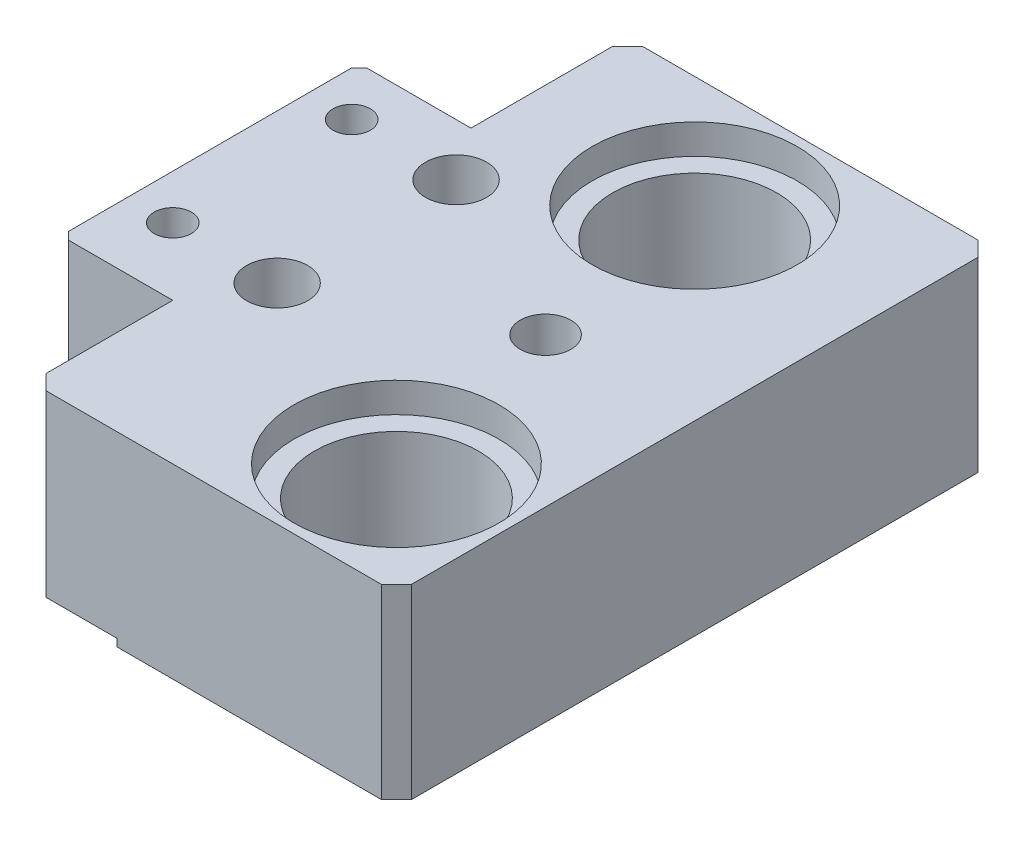
SolidWorks part; units mm, degrees
ref_plane "Front Plane" through (0, 0, 0) normal (0, 0, 1) x (1, 0, 0)
ref_plane "Top Plane" through (0, 0, 0) normal (0, 1, 0) x (1, 0, 0)
ref_plane "Right Plane" through (0, 0, 0) normal (1, 0, 0) x (0, 0, -1)
sketch "Sketch1" plane through (0, 0, 0) normal (0, 0, 1) x (1, 0, 0)
  line L0 (0, 91.2981) -> (0, -100.4583) construction
  line L1 (-32, 12.5) -> (32, 12.5)
  line L2 (-32, 12.5) -> (-32, -12.5)
  line L3 (-32, -12.5) -> (32, -12.5)
  line L4 (32, 12.5) -> (32, -12.5)
  line L5 (-125.8092, 0) -> (111.3632, 0) construction
  dimension "D1" = 64
  dimension "D2" = 25
extrude "Boss-Extrude1" add sketch "Sketch1" along normal mid plane 80
sketch "Sketch3" plane through (0, 12.5, 0) normal (0, 1, 0) x (1, 0, 0)
  line L0 (-32, -40) -> (32, -40) construction
  line L1 (32, -40) -> (32, 40) construction
  line L2 (-12, -12) -> (-12, 12) construction
  line L3 (-12, 0) -> (-32, 0) construction
  line L4 (-32, -40) -> (-32, 40) construction
  circle A0 centre (7, 25) radius 11
  circle A1 centre (17, -25) radius 11
  circle A2 centre (-12, 12) radius 2.5
  circle A3 centre (-12, -12) radius 2.5
  circle A4 centre (-26, 12) radius 2.5
  circle A5 centre (-26, -12) radius 2.5
  dimension "D1" = 22
  dimension "D2" = 15
  dimension "D3" = 15
  dimension "D4" = 22
  dimension "D5" = 10
  dimension "D6" = 50
  dimension "D8" = 5
  dimension "D10" = 6
  dimension "D7" = 24
  dimension "D9" = 20
extrude "Cut-Extrude1" cut sketch "Sketch3" against normal through all
hole_wizard "M3 Tapped Hole1" positions "Sketch5" profile "Sketch4" tap size "M3" standard "Gb"
sketch "Sketch5" plane through (-32, 0, 0) normal (-1, 0, 0) x (0, 0, 1)
  line L0 (0, -23.1259) -> (0, 24.6172) construction
  line L2 (40, -12.5) -> (-40, -12.5) construction
  point P0 (0, 3.5)
  point P1 (-6, -7.5)
  point P3 (6, -7.5)
  dimension "D1" = 5
  dimension "D2" = 11
  dimension "D3" = 12
sketch "Sketch4" plane through (-32, 3.5, 0) normal (0, 1, 0) x (0, 0, 1)
  line L0 (0, 0) -> (0, 8.2511)
  line L1 (0, 8.2511) -> (1.25, 7.5)
  line L2 (1.25, 7.5) -> (1.25, 0)
  line L5 (1.25, 0) -> (0, 0)
  line L10 (0, 8.2511) -> (-1.25, 7.5) construction
  line L11 (0, -6.35) -> (0, 107.95) construction
  dimension "螺纹孔钻头直径" = 2.5
  dimension "螺纹孔钻头深度" = 7.5
  dimension "导头角度" = 118
cosmetic thread "Hole cosmetic thread1" parameters "D1"=6, "D2"=3
cosmetic thread "Hole cosmetic thread2" parameters "D1"=6, "D2"=3
cosmetic thread "Hole cosmetic thread3" parameters "D1"=6, "D2"=3
hole_wizard "M8 Tapped Hole1" positions "Sketch8" profile "Sketch7" tap size "M8" standard "Gb"
sketch "Sketch8" plane through (0, 12.5, 0) normal (0, 1, 0) x (-1, 0, 0)
  line L0 (-32, 40) -> (-32, -40) construction
  point P0 (-12, 0)
  dimension "D1" = 20
sketch "Sketch7" plane through (12, 12.5, 0) normal (1, 0, 0) x (0, 0, 1)
  line L0 (0, 0) -> (0, 22.0429)
  line L1 (0, 22.0429) -> (3.4, 20)
  line L2 (3.4, 20) -> (3.4, 0)
  line L5 (3.4, 0) -> (0, 0)
  line L10 (0, 22.0429) -> (-3.4, 20) construction
  line L11 (0, -6.35) -> (0, 107.95) construction
  dimension "螺纹孔钻头直径" = 6.8
  dimension "螺纹孔钻头深度" = 20
  dimension "导头角度" = 118
cosmetic thread "Hole cosmetic thread4" parameters "D1"=16, "D2"=8
sketch "Sketch11" plane through (0, 12.5, 0) normal (0, 1, 0) x (1, 0, 0)
  line L1 (-32, 40) -> (-17, 40)
  line L2 (-32, 40) -> (-32, 19)
  line L3 (-32, 19) -> (-17, 19)
  line L4 (-17, 40) -> (-17, 19)
  line L5 (-32, -40) -> (-17, -40)
  line L6 (-32, -40) -> (-32, -21)
  line L7 (-32, -21) -> (-17, -21)
  line L8 (-17, -40) -> (-17, -21)
  dimension "D1" = 15
  dimension "D2" = 40
  dimension "D3" = 19
extrude "Cut-Extrude5" cut sketch "Sketch11" against normal through all
sketch "Sketch13" plane through (0, -12.5, 0) normal (0, -1, 0) x (1, 0, 0)
  line L0 (-26, 12) -> (-26, -12) construction
  circle A0 centre (-26, -12) radius 4
  circle A1 centre (-26, 12) radius 4
  circle A2 centre (-12, 12) radius 4
  circle A3 centre (-12, -12) radius 4
  circle A4 centre (-26, 0) radius 4.1
  dimension "D1" = 8
  dimension "D2" = 8.2
extrude "Cut-Extrude7" cut sketch "Sketch13" against normal blind 13
sketch "Sketch14" plane through (0, 12.5, 0) normal (0, 1, 0) x (1, 0, 0)
  circle A0 centre (-12, -12) radius 4.1
  circle A1 centre (-12, 12) radius 4.1
  dimension "D1" = 8.2
extrude "Cut-Extrude8" cut sketch "Sketch14" against normal blind 6
sketch "Sketch15" plane through (0, -12.5, 0) normal (0, -1, 0) x (-1, 0, 0)
  line L0 (17, 40) -> (-32, 40) construction
  line L1 (17, -40) -> (5.5, -40)
  line L2 (17, -40) -> (17, 40)
  line L3 (17, 40) -> (5.5, 40)
  line L4 (5.5, -40) -> (5.5, 40)
  line L5 (32, -21) -> (32, 19) construction
  line L6 (17, -40) -> (-32, -40) construction
  dimension "D1" = 15
  dimension "D2" = 11.5
extrude "Cut-Extrude11" cut sketch "Sketch15" against normal blind 1
sketch "Sketch16" plane through (0, 12.5, 0) normal (0, 1, 0) x (1, 0, 0)
  circle A0 centre (17, -25) radius 13.75
  circle A1 centre (7, 25) radius 13.75
  dimension "D1" = 27.5
  dimension "D2" = 27.5
extrude "Cut-Extrude12" cut sketch "Sketch16" against normal blind 4
chamfer "Chamfer2" distance 2 angle 45 4 edges at (32, 0, -40) (32, 0, 40) (-17, 0.5, 40) (-17, 0.5, -40)
chamfer "Chamfer3" distance 1 angle 45 2 edges at (-32, 0, -19) (-32, 0, 21)
